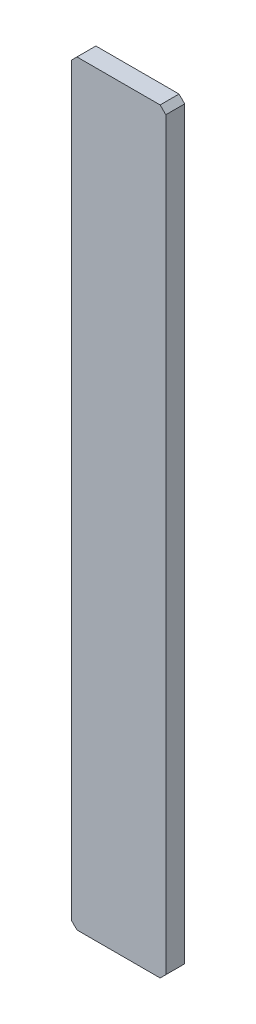
from build123d import *

# Parameters (mm, degrees)
SKETCH1_W           = 50
SKETCH1_H           = 400
BOSS_EXTRUDE1_DEPTH = 10
CHAMFER1_SIZE       = 3


with BuildPart() as part:
    # Sketch1 → Boss-Extrude1 (new body)
    with BuildSketch(Plane.XY):
        with Locations((-103.557058929, 349.193548387)):
            Rectangle(SKETCH1_W, SKETCH1_H)
    extrude(amount=BOSS_EXTRUDE1_DEPTH)

    # Chamfer1
    chamfer1_edges = [part.edges().sort_by_distance(p)[0] for p in [
        (-128.557058929, 549.193548387, 5),
        (-78.557058929, 549.193548387, 5),
        (-78.557058929, 149.193548387, 5),
        (-128.557058929, 149.193548387, 5),
    ]]
    chamfer(chamfer1_edges, length=CHAMFER1_SIZE)


solid = part.part
